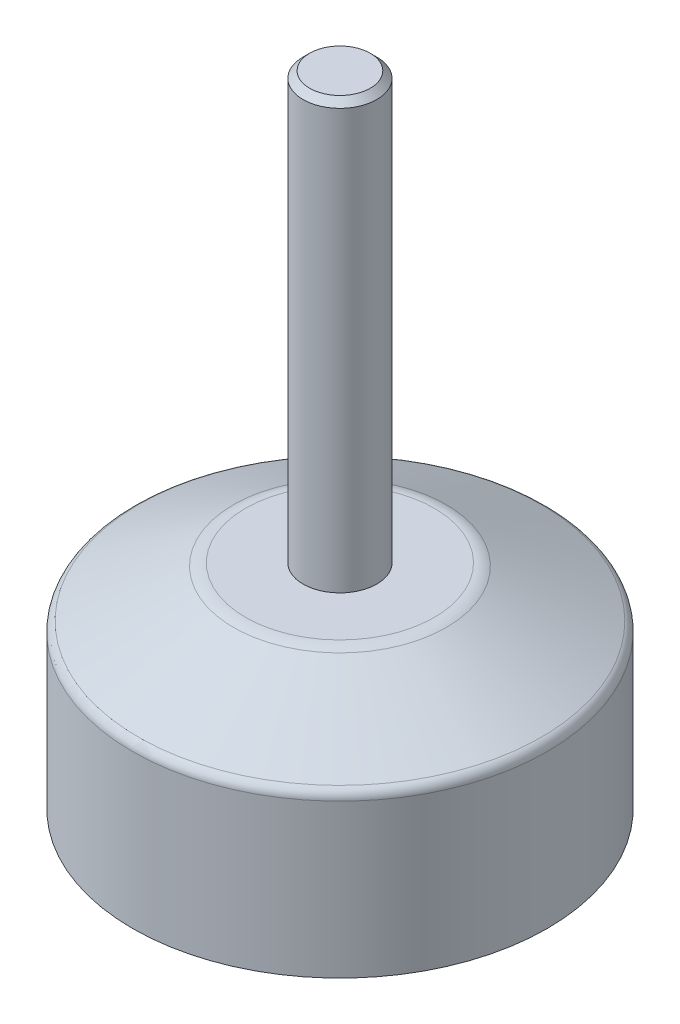
SolidWorks part; units mm, degrees
material "1060 合金"
ref_plane "前视基准面" through (0, 0, 0) normal (0, 0, 1) x (1, 0, 0)
ref_plane "上视基准面" through (0, 0, 0) normal (0, 1, 0) x (1, 0, 0)
ref_plane "右视基准面" through (0, 0, 0) normal (1, 0, 0) x (0, 0, -1)
other "Configuration Table"
ref_plane "基准面1" through (0, 0, 0) normal (0, 0, -1) x (-1, 0, 0)
sketch "草图1" plane through (0, 0, 0) normal (0, 0, -1) x (-1, 0, 0)
  line L0 (-20, -25) -> (-0.54, -25)
  line L1 (-0.54, -25) -> (-0.54, 35)
  line L2 (-0.54, 35) -> (-3.3865, 35)
  line L3 (-3.3865, 35) -> (-4, 34.3865)
  line L4 (-4, 34.3865) -> (-4, -5)
  line L5 (-4, -5) -> (-9.4098, -5)
  line L6 (-10.5279, -5.2639) -> (-19.4472, -9.7236)
  line L7 (-20, -10.618) -> (-20, -25)
  line L8 (-0.54, -25) -> (-0.54, 35) construction
  arc A0 (-9.4098, -5) -> (-10.5279, -5.2639) centre (-9.4098, -7.5) ccw
  arc A1 (-19.4472, -9.7236) -> (-20, -10.618) centre (-19, -10.618) ccw
  dimension "D1" = 3.46
  dimension "D2" = 60
  dimension "D3" = 20
revolve "旋转1" add sketch "草图1" angle 360 about L8
